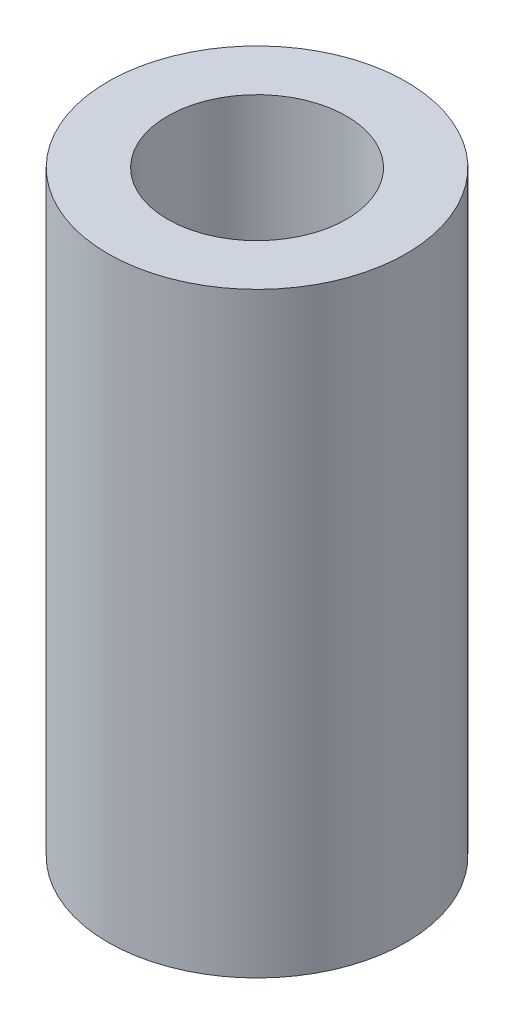
from build123d import *

# Parameters (mm, degrees)
SKETCH_1_R      = 2.5
SKETCH_1_R_2    = 1.5
EXTRUDE_1_DEPTH = 10


with BuildPart() as part:
    # 草图1 → 凸台-拉伸1 (new body)
    with BuildSketch(Plane(origin=(0, 0, 0), x_dir=(1, 0, 0), z_dir=(0, 1, 0))):
        with Locations(Location((0, 0, 0), (0, 0, 270))):
            Circle(SKETCH_1_R)
        with Locations(Location((0, 0, 0), (0, 0, 270))):
            Circle(SKETCH_1_R_2, mode=Mode.SUBTRACT)
    extrude(amount=EXTRUDE_1_DEPTH)


solid = part.part
